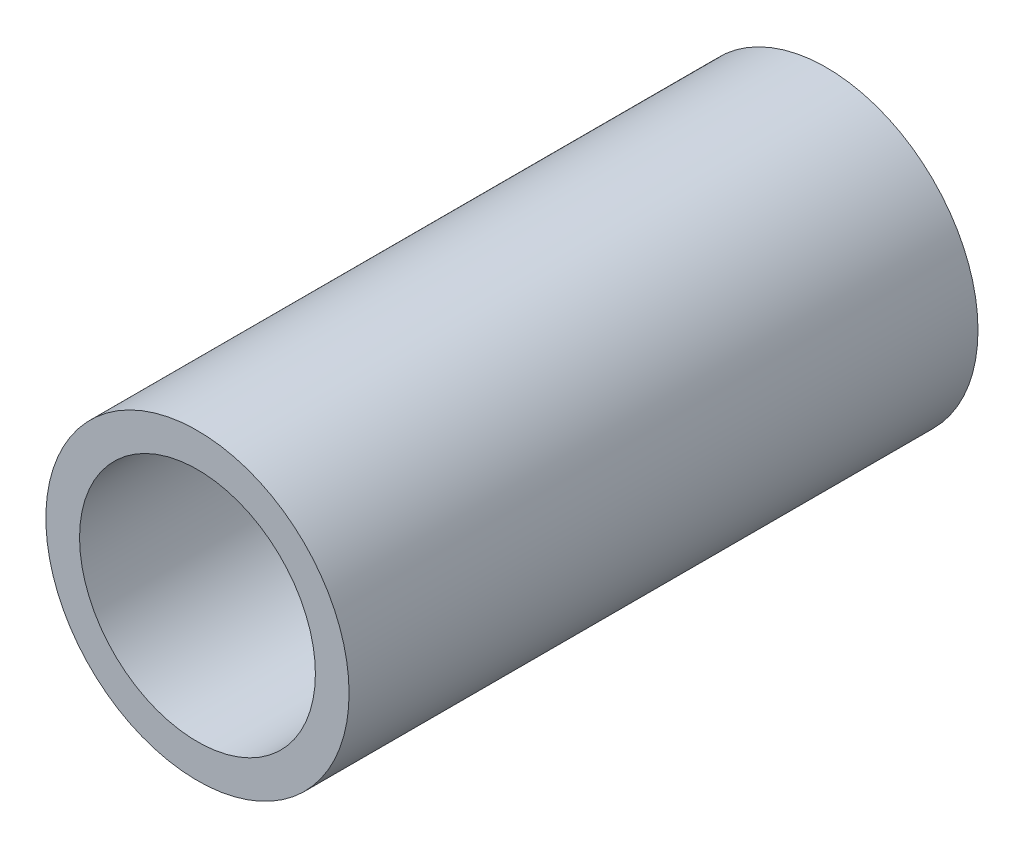
SolidWorks part; units mm, degrees
material "镀锌焊接钢管 Q215A"
ref_plane "Front Plane" through (0, 0, 0) normal (0, 0, 1) x (1, 0, 0)
ref_plane "Top Plane" through (0, 0, 0) normal (0, 1, 0) x (1, 0, 0)
ref_plane "Right Plane" through (0, 0, 0) normal (1, 0, 0) x (0, 0, -1)
sketch "Sketch1" plane through (0, 0, 0) normal (0, 0, 1) x (1, 0, 0)
  circle A0 centre (0, 0) radius 13.5
  circle A1 centre (0, 0) radius 10.5
  dimension "D1" = 3
  dimension "D2" = 21
extrude "Boss-Extrude1" add sketch "Sketch1" along normal mid plane 56
